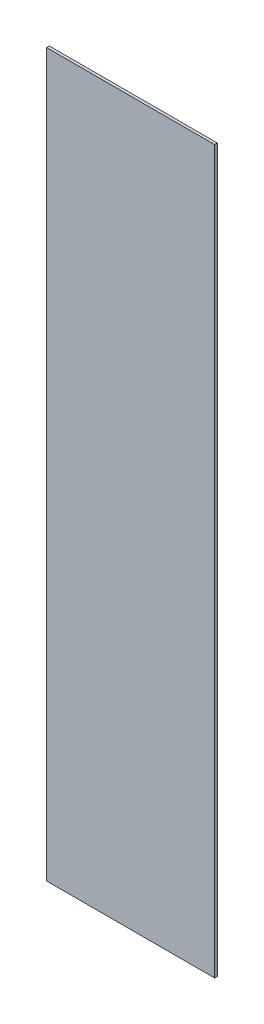
SolidWorks part; units mm, degrees
material "PMMA(有机玻璃)"
ref_plane "前视" through (0, 0, 0) normal (0, 0, 1) x (1, 0, 0)
ref_plane "上视" through (0, 0, 0) normal (0, 1, 0) x (1, 0, 0)
ref_plane "右视" through (0, 0, 0) normal (1, 0, 0) x (0, 0, -1)
sketch "草图1" plane through (0, 0, 0) normal (0, 0, 1) x (1, 0, 0)
  line L1 (-152, 653) -> (152, 653)
  line L2 (-152, 653) -> (-152, -653)
  line L3 (-152, -653) -> (152, -653)
  line L4 (152, 653) -> (152, -653)
  line L5 (-152, 653) -> (152, -653) construction
  line L6 (-152, -653) -> (152, 653) construction
  point P0 (0, 0)
  dimension "D1" = 1306
  dimension "D2" = 304
extrude "凸台-拉伸1" add sketch "草图1" along normal blind 5
hole_wizard "M5 间隙孔1" positions "草图3" profile "草图2" hole size "M5" standard "GB"
sketch "草图3" plane through (0, 0, 5) normal (0, 0, 1) x (1, 0, 0)
  line L0 (-427.5, 273) -> (-427.5, -273) construction
  line L1 (-427.5, -273) -> (427.5, -273) construction
  line L2 (0, 273) -> (0, -273) construction
  line L3 (427.5, 273) -> (-427.5, 273) construction
  line L5 (-427.5, 0) -> (427.5, 0) construction
  line L6 (427.5, -273) -> (427.5, 273) construction
  point P0 (-375, -261)
  point P46 (415.5, 250)
  point P48 (-415.5, 250)
  point P58 (-125, -261)
  point P59 (125, -261)
  point P61 (-125, 261)
  point P62 (125, 261)
  point P64 (-375, 261)
  point P88 (375, -261)
  point P89 (375, 261)
  point P108 (415.5, 0)
  point P109 (-415.5, 0)
  point P110 (415.5, -250)
  point P111 (-415.5, -250)
  dimension "D1" = 12
  dimension "D2" = 12
  dimension "D5" = 3
  dimension "D3" = 12
  dimension "D6" = 4
  dimension "D4" = 2
sketch "草图2" plane through (-375, -261, 5) normal (1, 0, 0) x (0, -1, 0)
  line L0 (0, 0) -> (0, 5)
  line L1 (0, 5) -> (2.75, 5)
  line L2 (2.75, 5) -> (2.75, 0)
  line L5 (2.75, 0) -> (0, 0)
  line L11 (0, -6.35) -> (0, 107.95) construction
  dimension "通孔孔直径" = 5.5
  dimension "通孔孔深度" = 5
